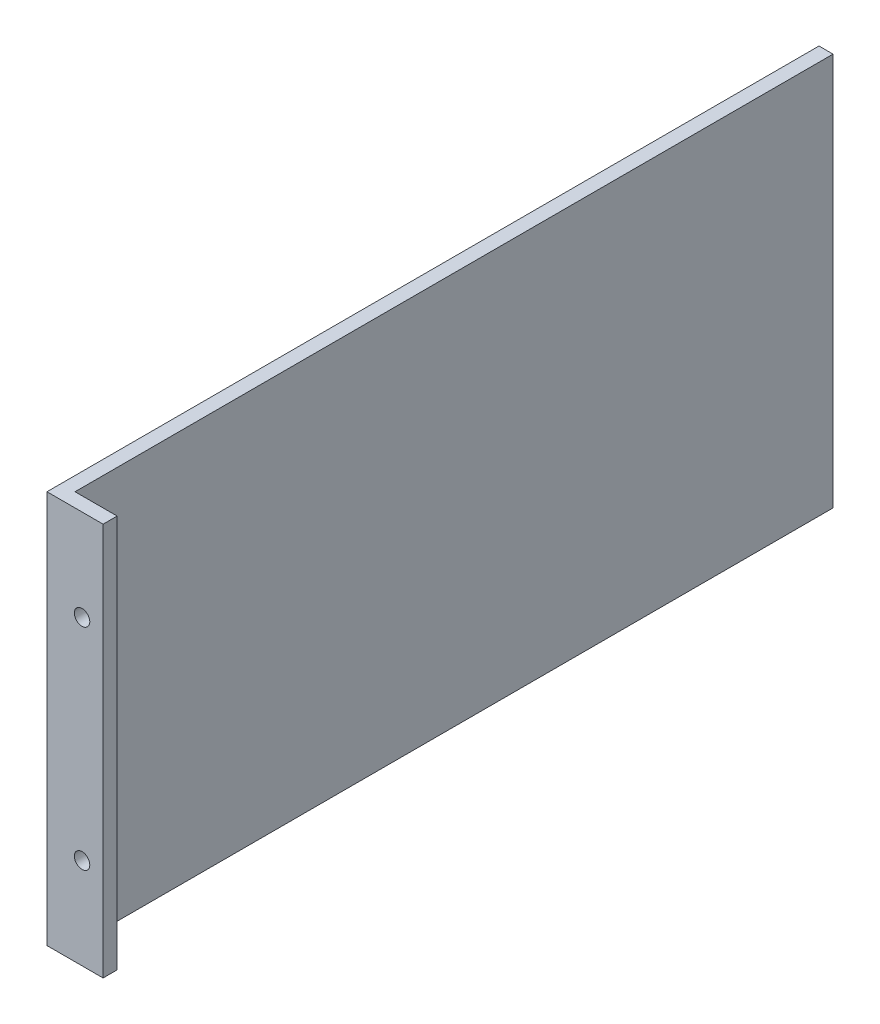
from build123d import *

# Parameters (mm, degrees)
BOSS_EXTRUDE1_DEPTH = 1100
CUT_EXTRUDE1_DEPTH  = 1295.604186615
SKETCH3_W           = 20
SKETCH3_H           = 560
BOSS_EXTRUDE2_DEPTH = 60
SKETCH4_R           = 11
CUT_EXTRUDE2_DEPTH  = 1288.953803519


with BuildPart() as part:
    # Sketch1 → Boss-Extrude1 (new body)
    with BuildSketch(Plane.XY):
        Polygon((360, 0), (-360, 0), (-360, 20), (-335, 20), (-335, 580), (-315, 580), (-315, 20), (315, 20), (315, 580), (335, 580), (335, 20), (360, 20), align=None)
    extrude(amount=BOSS_EXTRUDE1_DEPTH)

    # Sketch2 → Cut-Extrude1 (cut, through all)
    with BuildSketch(Plane(origin=(0, 0, 0), x_dir=(-1, 0, 0), z_dir=(0, 0, -1))):
        Polygon((-360, 20), (-59.240800915, 20), (-59.240800915, 755.063041929), (647.427412598, 706.251760561), (560.651801276, -150.657401245), (-360, -188.621731198), (-684.035873625, -70.661134557), align=None)
    extrude(amount=-CUT_EXTRUDE1_DEPTH, mode=Mode.SUBTRACT)

    # Sketch3 → Boss-Extrude2 (add)
    with BuildSketch(Plane(origin=(335, 0, 0), x_dir=(0, 0, -1), z_dir=(1, 0, 0))):
        with Locations((-1090, 300)):
            Rectangle(SKETCH3_W, SKETCH3_H)
    extrude(amount=BOSS_EXTRUDE2_DEPTH)

    # Sketch4 → Cut-Extrude2 (cut, through all)
    with BuildSketch(Plane(origin=(0, 0, 1080), x_dir=(-1, 0, 0), z_dir=(0, 0, -1))):
        with Locations((-365, 450)):
            Circle(SKETCH4_R)
        with Locations((-365, 150)):
            Circle(SKETCH4_R)
    extrude(amount=-CUT_EXTRUDE2_DEPTH, mode=Mode.SUBTRACT)


solid = part.part
